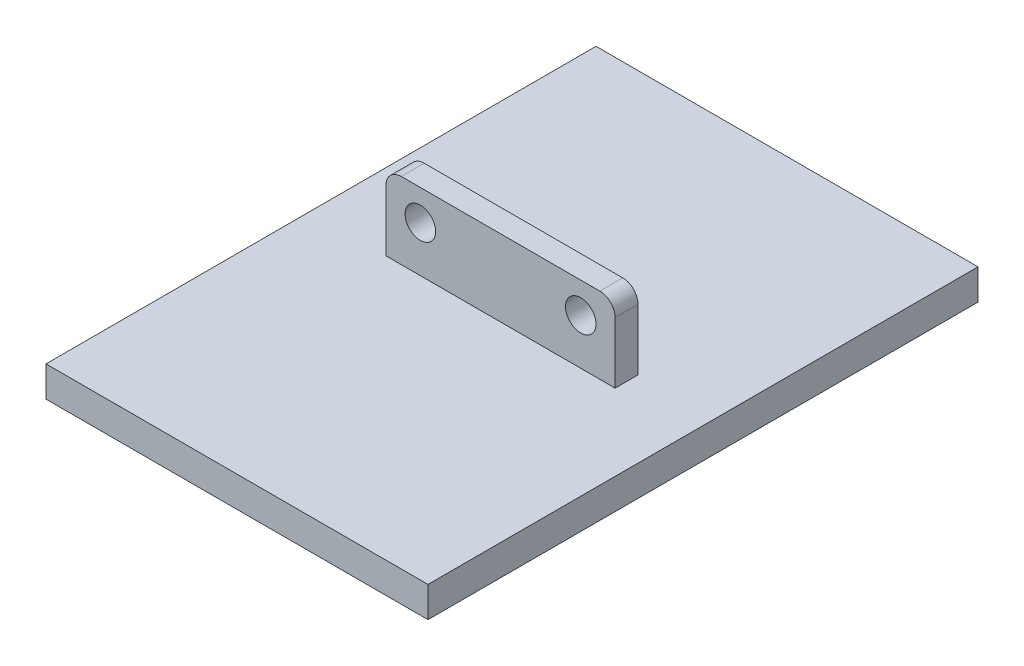
SolidWorks part; units mm, degrees
ref_plane "Front Plane" through (0, 0, 0) normal (0, 0, 1) x (1, 0, 0)
ref_plane "Top Plane" through (0, 0, 0) normal (0, 1, 0) x (1, 0, 0)
ref_plane "Right Plane" through (0, 0, 0) normal (1, 0, 0) x (0, 0, -1)
sketch "Sketch1" plane through (0, 0, 0) normal (0, 1, 0) x (1, 0, 0)
  line L1 (-125, 180) -> (125, 180)
  line L2 (-125, 180) -> (-125, -180)
  line L3 (-125, -180) -> (125, -180)
  line L4 (125, 180) -> (125, -180)
  line L5 (-125, 180) -> (125, -180) construction
  line L6 (-125, -180) -> (125, 180) construction
  point P0 (0, 0)
  dimension "D1" = 250
  dimension "D2" = 360
extrude "Boss-Extrude1" add sketch "Sketch1" along normal blind 20
sketch "Sketch2" plane through (0, 20, 0) normal (0, 1, 0) x (1, 0, 0)
  line L1 (75, 7.5) -> (-75, 7.5)
  line L2 (75, 7.5) -> (75, -7.5)
  line L3 (75, -7.5) -> (-75, -7.5)
  line L4 (-75, 7.5) -> (-75, -7.5)
  line L5 (75, 7.5) -> (-75, -7.5) construction
  line L6 (75, -7.5) -> (-75, 7.5) construction
  point P0 (0, 0)
  dimension "D1" = 15
  dimension "D2" = 150
extrude "Boss-Extrude2" add sketch "Sketch2" along normal blind 50
fillet "Fillet1" radius 10 2 edges at (-75, 70, 0) (75, 70, 0)
sketch "Sketch3" plane through (0, 0, 7.5) normal (0, 0, 1) x (1, 0, 0)
  line L0 (0, 0) -> (0, 115.6095) construction
  line L1 (-125, 0) -> (125, 0) construction
  line L2 (-65, 70) -> (65, 70) construction
  circle A0 centre (52.5, 50) radius 10
  circle A1 centre (-52.5, 50) radius 10
  dimension "D1" = 105
  dimension "D3" = 20
  dimension "D2" = 20
extrude "Cut-Extrude1" cut sketch "Sketch3" against normal through all
